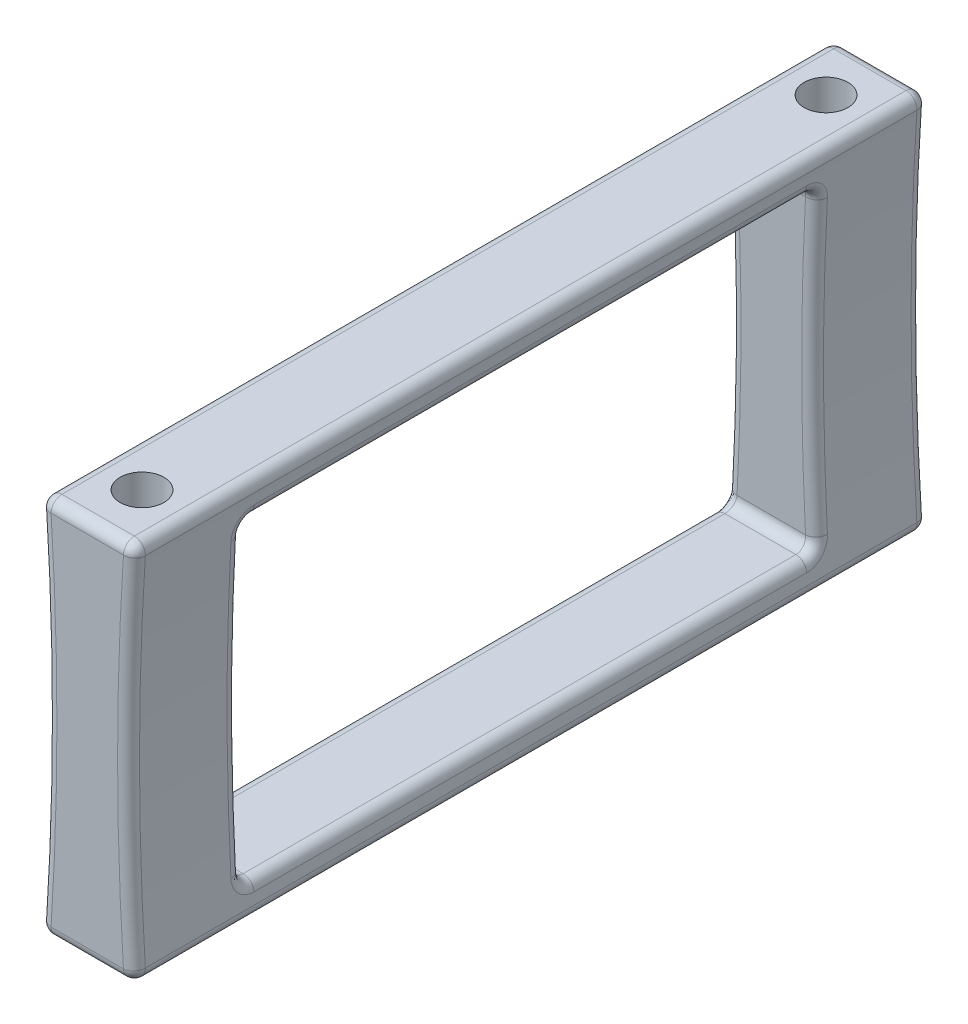
SolidWorks part; units mm, degrees
material "PA 类型 6"
ref_plane "前视基准面" through (0, 0, 0) normal (0, 0, 1) x (1, 0, 0)
ref_plane "上视基准面" through (0, 0, 0) normal (0, 1, 0) x (1, 0, 0)
ref_plane "右视基准面" through (0, 0, 0) normal (1, 0, 0) x (0, 0, -1)
other "Configuration Table"
sketch "草图1" plane through (0, 0, 0) normal (0, 0, 1) x (1, 0, 0)
  line L0 (0, 0) -> (0, 13.9) construction
  line L1 (-3.5, 13.9) -> (3.5, 13.9)
  line L2 (-3.5, 13.9) -> (-3.5, -13.9) construction
  line L3 (-3.5, -13.9) -> (3.5, -13.9)
  line L4 (3.5, 13.9) -> (3.5, -13.9) construction
  line L5 (-3.5, 13.9) -> (3.5, -13.9) construction
  line L6 (-3.5, -13.9) -> (3.5, 13.9) construction
  line L7 (1.5, 13.9) -> (1.5, -13.9) construction
  arc A0 (3.5, 13.9) -> (3.5, -13.9) centre (203.5, 0) ccw
  arc A1 (-3.5, 13.9) -> (-3.5, -13.9) centre (-203.5, 0) cw
  point P0 (0, 0)
  dimension "D3" = 200
  dimension "D1" = 27.8
  dimension "D2" = 7
  dimension "D4" = 1.5
extrude "凸台-拉伸1" add sketch "草图1" along normal blind 58
sketch "草图2" plane through (0, 0, 0) normal (1, 0, 0) x (0, 0, -1)
  line L0 (0, 0) -> (-71.1257, 0) construction
  line L1 (0, -13.9) -> (0, 13.9) construction
  line L2 (-50, 11.5) -> (-8, 11.5)
  line L3 (-50, 11.5) -> (-50, -11.5)
  line L4 (-50, -11.5) -> (-8, -11.5)
  line L5 (-8, 11.5) -> (-8, -11.5)
  line L6 (-50, 11.5) -> (-8, -11.5) construction
  line L7 (-50, -11.5) -> (-8, 11.5) construction
  line L8 (-58, 13.9) -> (-58, -13.9) construction
  point P3 (-29, 0)
  dimension "D1" = 8
  dimension "D2" = 23
  dimension "D3" = 8
extrude "切除-拉伸1" cut sketch "草图2" against normal through all both and the other way through all
sketch "草图3" plane through (0, 13.9, 0) normal (0, 1, 0) x (1, 0, 0)
  line L0 (0, 0) -> (0, -68.5032) construction
  line L1 (3.5, 0) -> (-3.5, 0) construction
  line L2 (3.5, -58) -> (-3.5, -58) construction
  line L3 (3.0176, -8) -> (3.3477, -8) construction
  circle A0 centre (0, -4) radius 1.6
  circle A1 centre (0, -54) radius 1.6
  dimension "D1" = 3.2
  dimension "D2" = 4
  dimension "D3" = 4
extrude "切除-拉伸2" cut sketch "草图3" against normal through all
fillet "圆角1" radius 0.8 24 edges at (-3.3477, 11.5, 29) (-3.3477, -11.5, 29) (3.3477, -11.5, 29) (3.3477, 11.5, 29) (0, -13.9, 0) (3.0176, 0, 0) (0, 13.9, 0) (-3.0176, 0, 0) (0, 13.9, 58) (3.0176, 0, 58) (0, -13.9, 58) (-3.0176, 0, 58) (-3.0176, 0, 50) (0, -11.5, 50) (3.0176, 0, 50) (0, 11.5, 50) (3.5, 13.9, 29) (-3.5, 13.9, 29) (-3.5, -13.9, 29) (3.5, -13.9, 29) (-3.0176, 0, 8) (0, 11.5, 8) (3.0176, 0, 8) (0, -11.5, 8)
